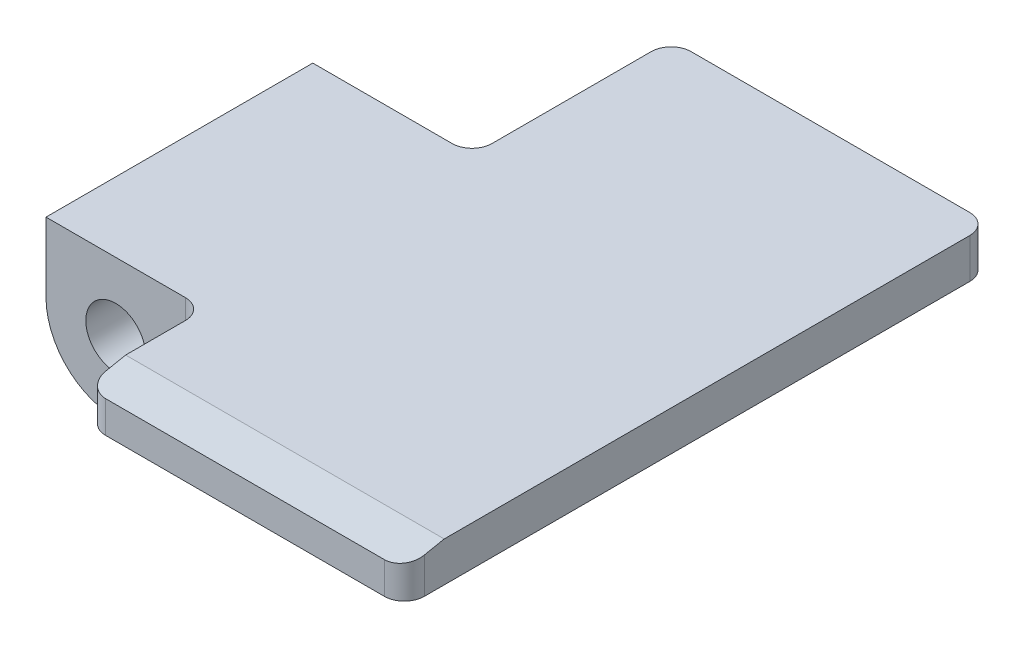
SolidWorks part; units mm, degrees
ref_plane "Front Plane" through (0, 0, 0) normal (0, 0, 1) x (1, 0, 0)
ref_plane "Top Plane" through (0, 0, 0) normal (0, 1, 0) x (1, 0, 0)
ref_plane "Right Plane" through (0, 0, 0) normal (1, 0, 0) x (0, 0, -1)
sketch "Sketch1" plane through (0, 0, 0) normal (0, 0, 1) x (1, 0, 0)
  circle A0 centre (0, 0) radius 1.75
  dimension "D1" = 3.5
extrude "Boss-Extrude1" add sketch "Sketch1" along normal blind 6.7
sketch "Sketch2" plane through (0, 0, 6.7) normal (0, 0, 1) x (1, 0, 0)
  circle A0 centre (0, 0) radius 0.75
  dimension "D1" = 1.5
extrude "Cut-Extrude1" cut sketch "Sketch2" against normal through all
ref_plane "Plane1" through (0, 1.75, 0) normal (0, 1, 0) x (1, 0, 0)
sketch "Sketch3" plane through (0, 1.75, 0) normal (0, 1, 0) x (1, 0, 0)
  line L1 (-1.75, 0) -> (10.25, 0)
  line L2 (-1.75, 0) -> (-1.75, -6.7)
  line L3 (-1.75, -6.7) -> (10.25, -6.7)
  line L4 (10.25, 0) -> (10.25, -6.7)
  dimension "D1" = 12
extrude "Boss-Extrude2" add sketch "Sketch3" against normal blind 1
sketch "Sketch4" plane through (0, 0, 6.7) normal (0, 0, 1) x (1, 0, 0)
  line L0 (-1.75, 0.75) -> (-1.75, 0)
  line L1 (-1.5811, 0.75) -> (-1.75, 0.75)
  arc A0 (-1.5811, 0.75) -> (1.5811, 0.75) centre (0, 0) ccw construction
  arc A1 (-1.5811, 0.75) -> (-1.75, 0) centre (0, 0) ccw
extrude "Boss-Extrude3" add sketch "Sketch4" against normal up to surface (6.7 mm away) up to face at (0.75, 0, 0)
sketch "Sketch5" plane through (0, 0, 6.7) normal (0, 0, 1) x (1, 0, 0)
  line L0 (1.5811, 0.75) -> (10.25, 0.75) construction
  line L1 (10.25, 1.75) -> (2.25, 1.75)
  line L2 (10.25, 1.75) -> (10.25, 0.75)
  line L3 (10.25, 0.75) -> (2.25, 0.75)
  line L4 (2.25, 1.75) -> (2.25, 0.75)
  dimension "D1" = 8
extrude "Boss-Extrude4" add sketch "Sketch5" along normal blind 3
sketch "Sketch6" plane through (0, 0, 0) normal (0, 0, -1) x (-1, 0, 0)
  line L4 (-2.25, 1.75) -> (-10.25, 1.75)
  line L5 (-2.25, 0.75) -> (-2.25, 1.75)
  line L6 (-10.25, 0.75) -> (-2.25, 0.75)
  line L7 (-10.25, 1.75) -> (-10.25, 0.75)
  line L8 (-2.25, 1.75) -> (-10.25, 1.75)
  line L9 (-2.25, 0.75) -> (-2.25, 1.75)
  line L10 (-10.25, 0.75) -> (-2.25, 0.75)
  line L11 (-10.25, 1.75) -> (-10.25, 0.75)
  dimension "D1" = 0
extrude "Boss-Extrude5" add sketch "Sketch6" along normal blind 5
chamfer "Chamfer1" distance 1 distance2 0.2 1 edges at (6.25, 1.75, 9.7)
fillet "Fillet1" radius 0.5 6 edges at (2.25, 1.25, 6.7) (2.25, 1.25, 0) (2.25, 1.25, -5) (10.25, 1.15, 9.7) (2.25, 1.15, 9.7) (10.25, 1.25, -5)
